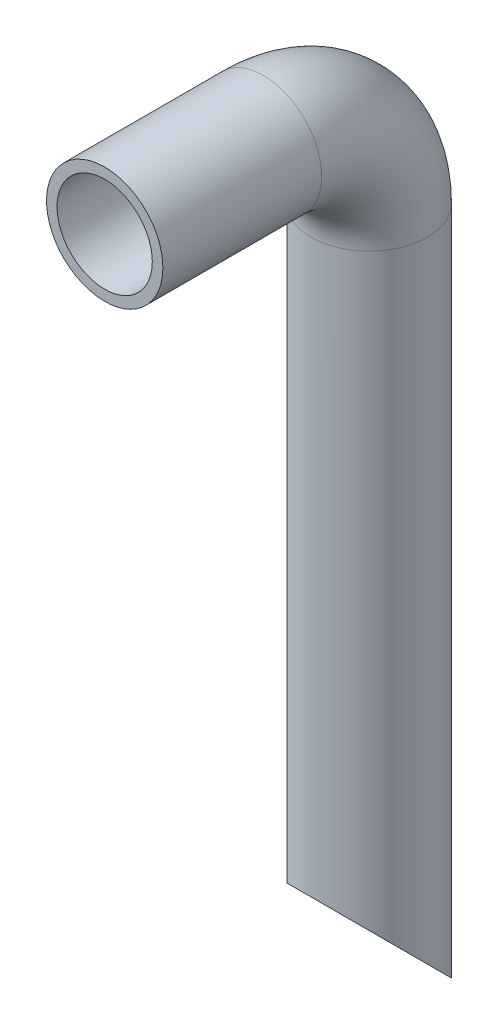
from build123d import *

# Parameters (mm, degrees)
SKETCH1_R          = 11
SKETCH1_R_2        = 9
CUT_EXTRUDE1_DEPTH = 25


with BuildPart() as part:
    # Sweep1: sweep along a path in Sketch2
    with BuildLine(Plane(origin=(0, 0, 0), x_dir=(0, 0, -1), z_dir=(1, 0, 0))) as sweep1_path:
        Line((0, 0), (30, 0))
        ThreePointArc((30, 0), (44.142135624, -5.857864376), (50, -20))
        Line((50, -20), (50, -150))
    # Sketch1 → Sweep1 (sweep)
    with BuildSketch(Plane.XY):
        Circle(SKETCH1_R)
        Circle(SKETCH1_R_2, mode=Mode.SUBTRACT)
    sweep(path=sweep1_path.line)

    # Sketch3 → Cut-Extrude1 (cut, symmetric)
    with BuildSketch(Plane(origin=(0, 0, 0), x_dir=(0, 0, -1), z_dir=(1, 0, 0))):
        Polygon((61, -150), (36.244444784, -125.244444784), (36.244444784, -150), align=None)
    extrude(amount=CUT_EXTRUDE1_DEPTH, both=True, mode=Mode.SUBTRACT)


solid = part.part
